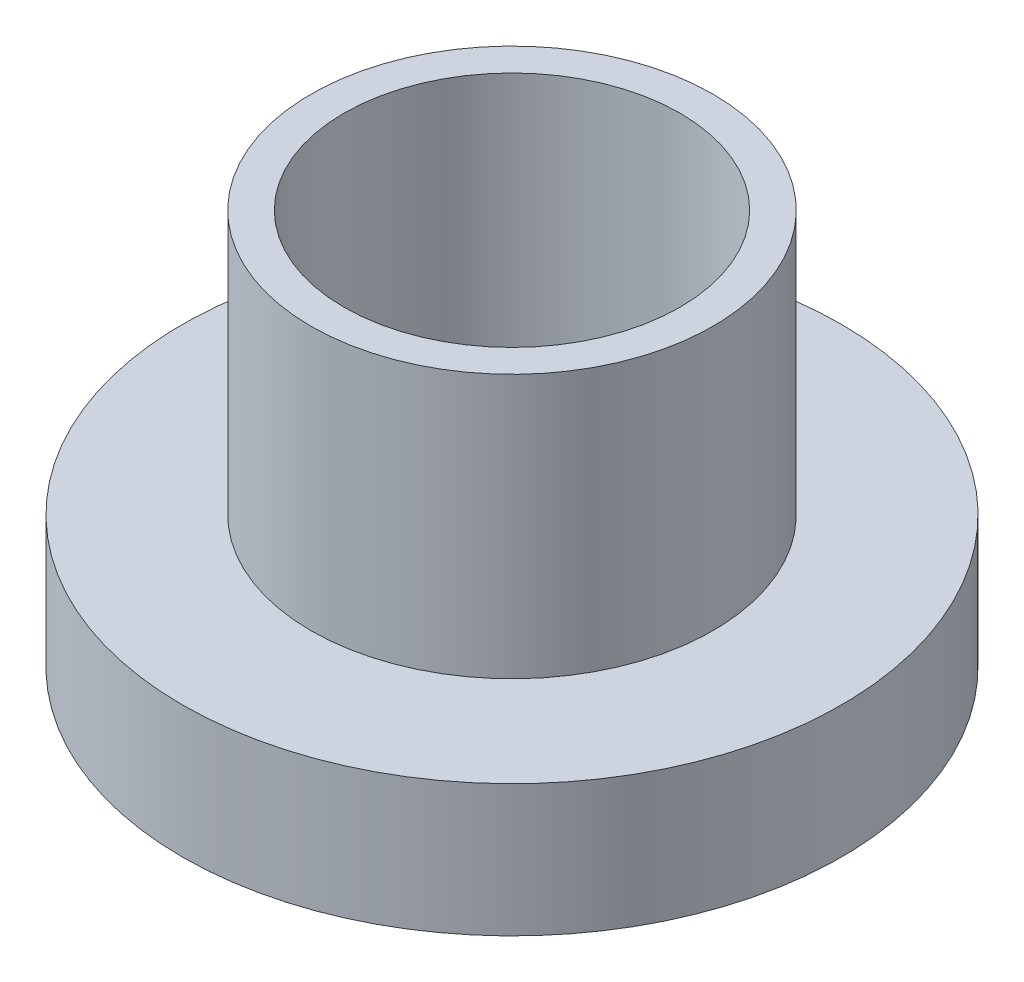
from build123d import *


with BuildPart() as part:
    # Sketch1 → Revolve1 (revolve)
    with BuildSketch(Plane.XY, mode=Mode.PRIVATE) as revolve1_sk:
        Polygon((25.5, 60), (25.5, 20), (12.5, 20), (12.5, 0), (50, 0), (50, 20), (30.5, 20), (30.5, 60), align=None)
    revolve(revolve1_sk.sketch.rotate(Axis((0, 0, 0), (0, 1, 0)), 90), axis=Axis((0, 0, 0), (0, 1, 0)))


solid = part.part
